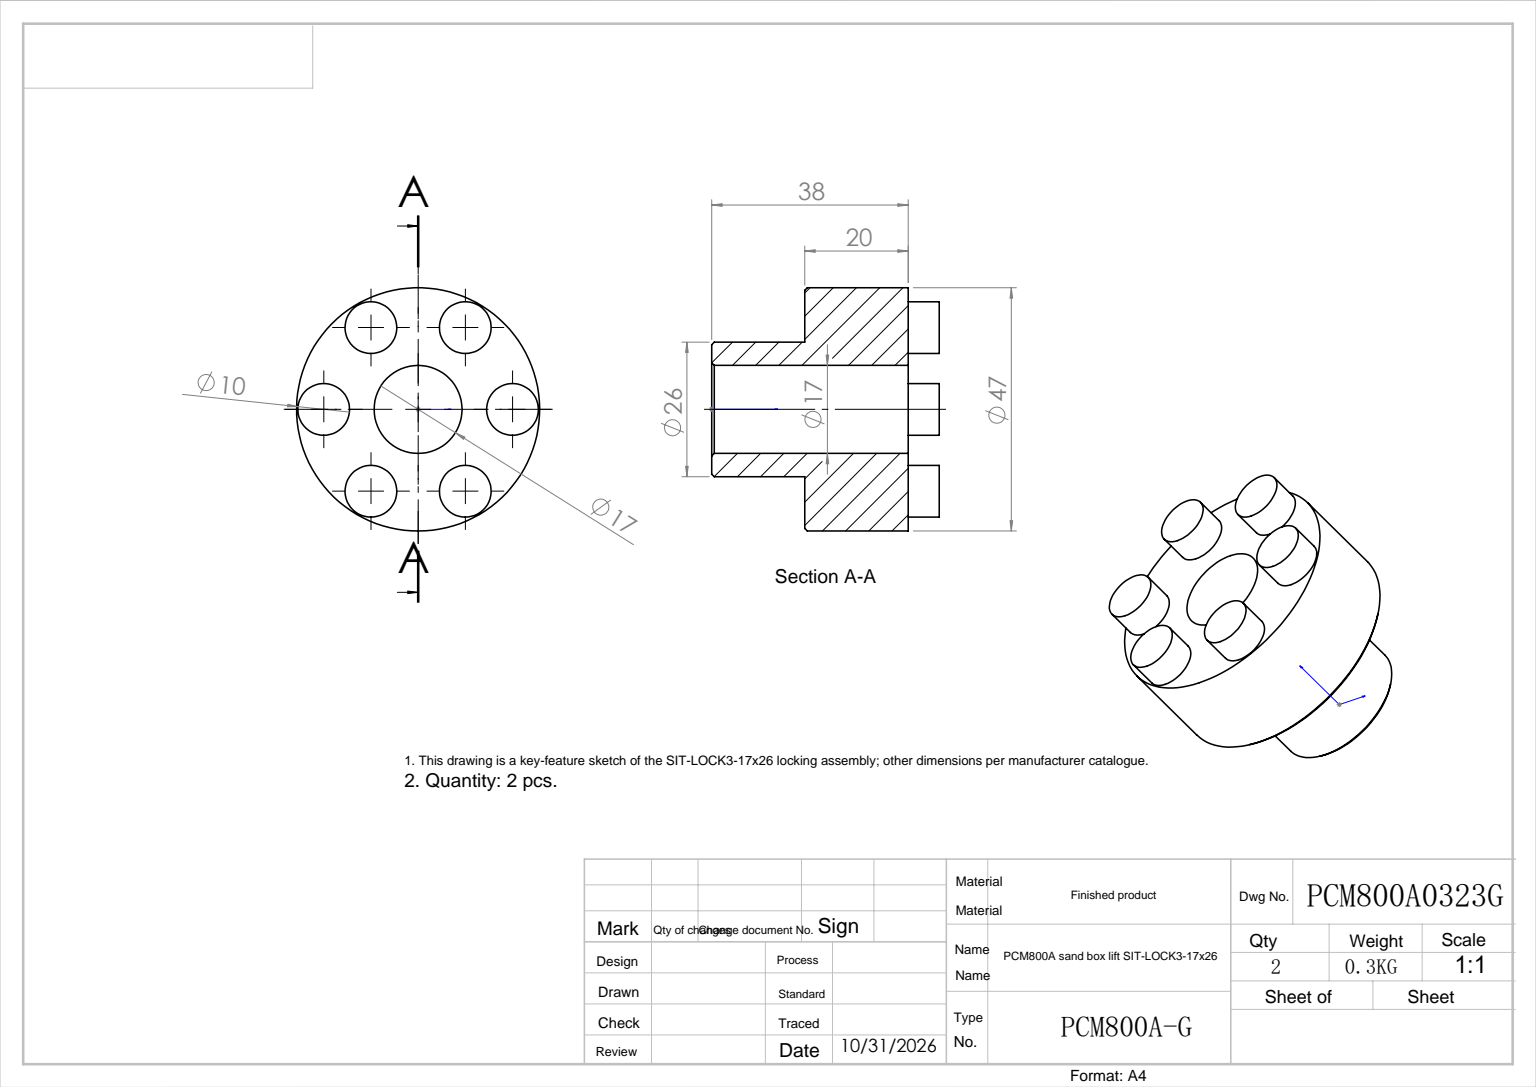
SolidWorks part; units mm, degrees
ref_plane "前视基准面" through (0, 0, 0) normal (0, 0, 1) x (1, 0, 0)
ref_plane "上视基准面" through (0, 0, 0) normal (0, 1, 0) x (1, 0, 0)
ref_plane "右视基准面" through (0, 0, 0) normal (1, 0, 0) x (0, 0, -1)
sketch "草图1" plane through (0, 0, 0) normal (0, 1, 0) x (1, 0, 0)
  circle A0 centre (0, 0) radius 8.5
  circle A1 centre (0, 0) radius 13
extrude "拉伸1" add sketch "草图1" along normal blind 18
sketch "草图2" plane through (0, 18, 0) normal (0, 1, 0) x (-1, 0, 0)
  circle A0 centre (0, 0) radius 23.5
extrude "拉伸2" add sketch "草图2" along normal blind 20
sketch "草图3" plane through (0, 18, 0) normal (0, -1, 0) x (1, 0, 0)
  circle A0 centre (0, 0) radius 8.5
extrude "切除-拉伸1" cut sketch "草图3" against normal through all
sketch "草图4" plane through (0, 38, 0) normal (0, 1, 0) x (-1, 0, 0)
  circle A0 centre (0, 0) radius 18.25 construction
  circle A1 centre (-18.25, 0) radius 5
  circle A2 centre (-9.125, 15.805) radius 5
  circle A3 centre (9.125, 15.805) radius 5
  circle A4 centre (18.25, 0) radius 5
  circle A5 centre (9.125, -15.805) radius 5
  circle A6 centre (-9.125, -15.805) radius 5
extrude "拉伸3" add sketch "草图4" along normal blind 6
chamfer "倒角1" distance 0.5 angle 45 3 edges at (0, 18, 23.5) (0, 0, 13) (0, 0, 8.5)
